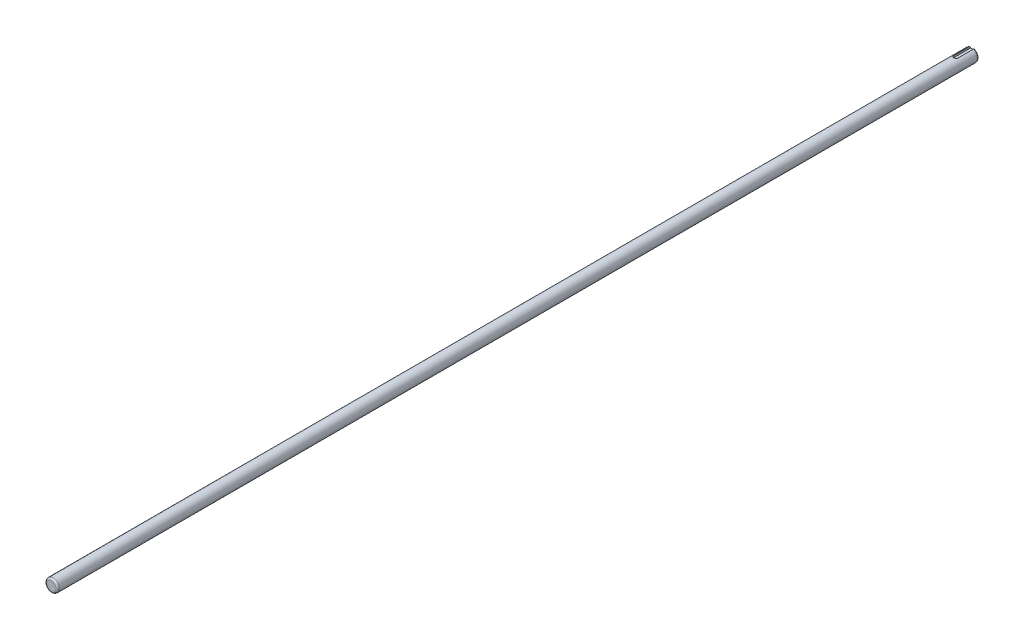
from build123d import *

# Parameters (mm, degrees)
SKETCH_1_R          = 7.5
EXTRUDE_1_DEPTH     = 545
FILLET_1_R          = 2
SKETCH_2_W          = 5
SKETCH_2_H          = 6.769617338
CUT_EXTRUDE_2_DEPTH = 20
SKETCH_3_R          = 2.5
CUT_EXTRUDE_3_DEPTH = 546.194919376


with BuildPart() as part:
    # 草图1 → 拉伸1 (new, symmetric)
    with BuildSketch(Plane.XY):
        Circle(SKETCH_1_R)
    extrude(amount=EXTRUDE_1_DEPTH, both=True)

    # 圆角1
    fillet_1_edges = [part.edges().sort_by_distance(p)[0] for p in [
        (-7.5, 0, -545),
        (-7.5, 0, 545),
    ]]
    fillet(fillet_1_edges, radius=FILLET_1_R)

    # 草图2 → 拉伸2 (cut)
    with BuildSketch(Plane(origin=(0, 0, -545), x_dir=(-1, 0, 0), z_dir=(0, 0, -1))):
        with Locations((0, 8.384808669)):
            Rectangle(SKETCH_2_W, SKETCH_2_H)
    extrude(amount=-CUT_EXTRUDE_2_DEPTH, mode=Mode.SUBTRACT)

    # 草图3 → 拉伸3 (cut, through all)
    with BuildSketch(Plane(origin=(0, 5, 0), x_dir=(1, 0, 0), z_dir=(0, 1, 0))):
        with Locations((0, 525)):
            Circle(SKETCH_3_R)
    extrude(amount=CUT_EXTRUDE_3_DEPTH, mode=Mode.SUBTRACT)


solid = part.part
